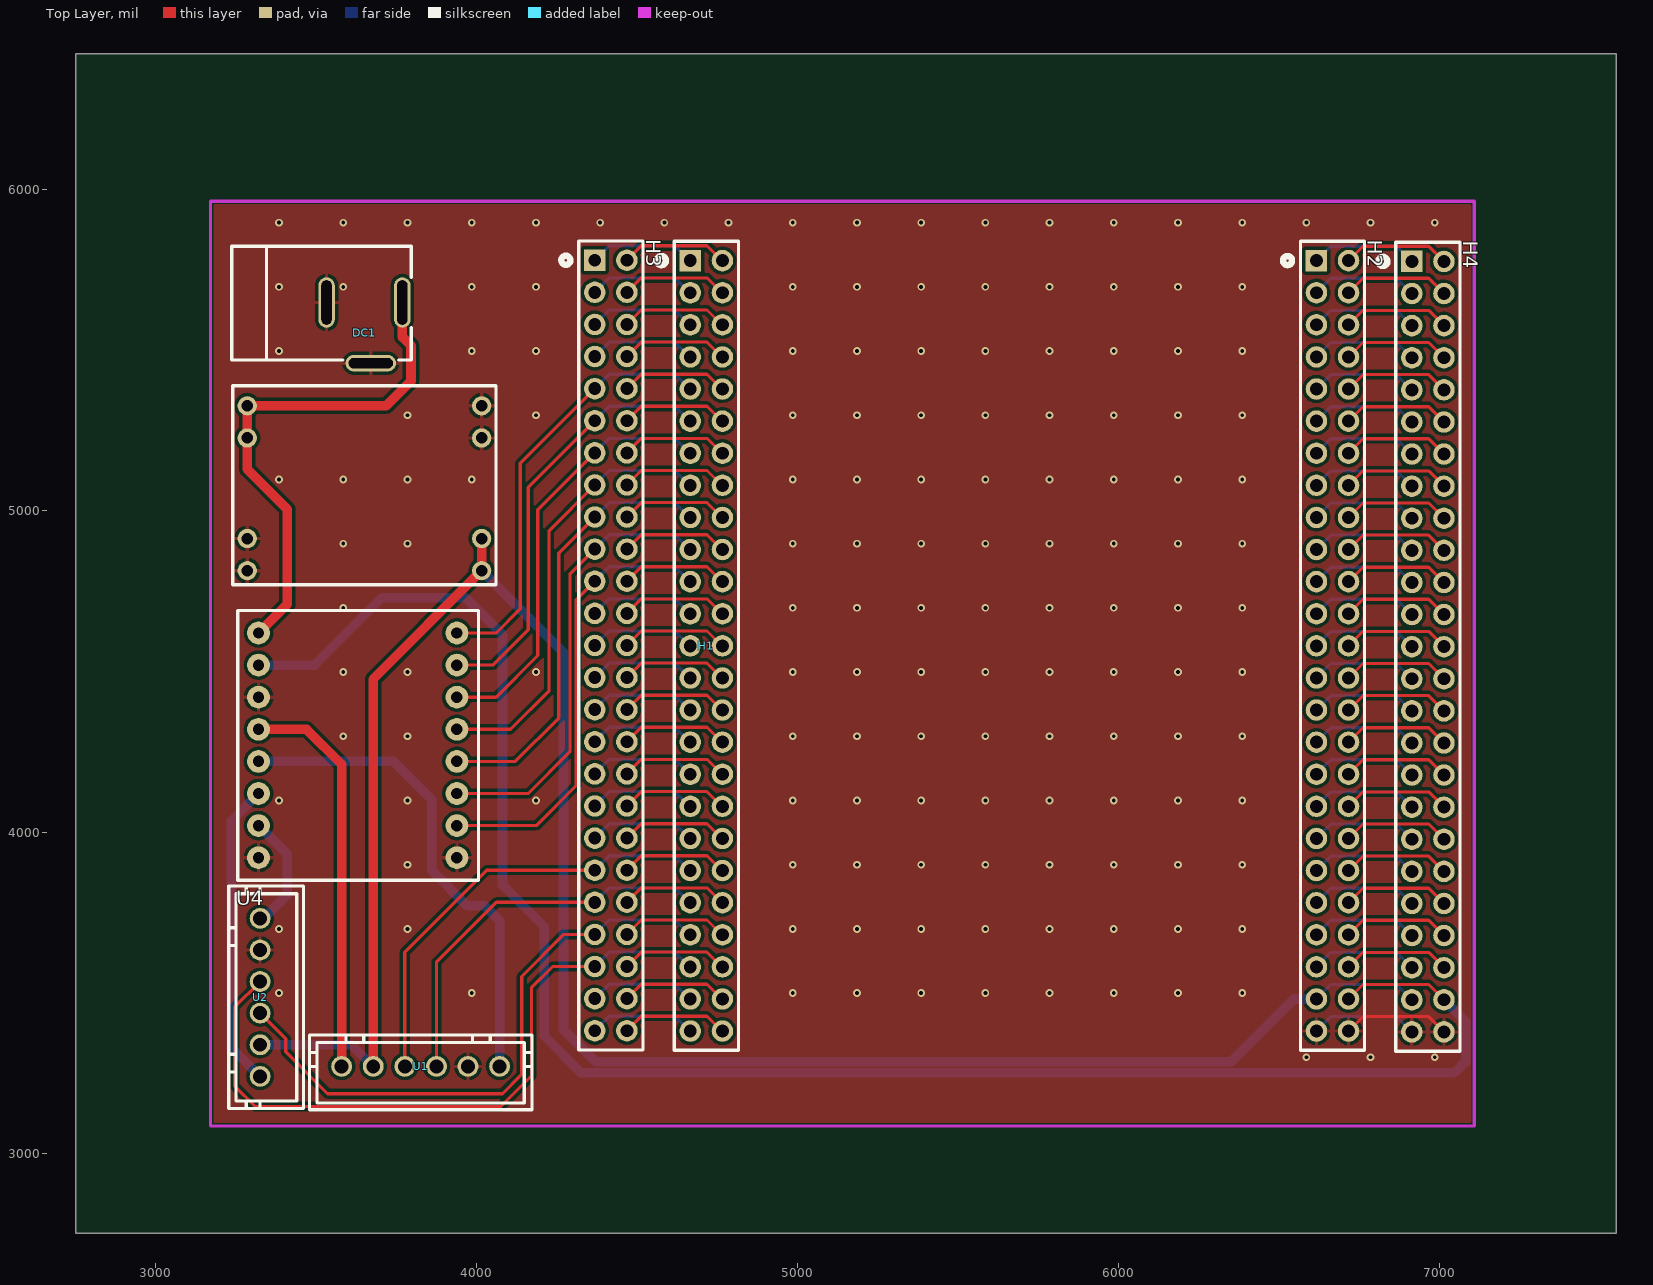
[diagram p0: Top Layer view]
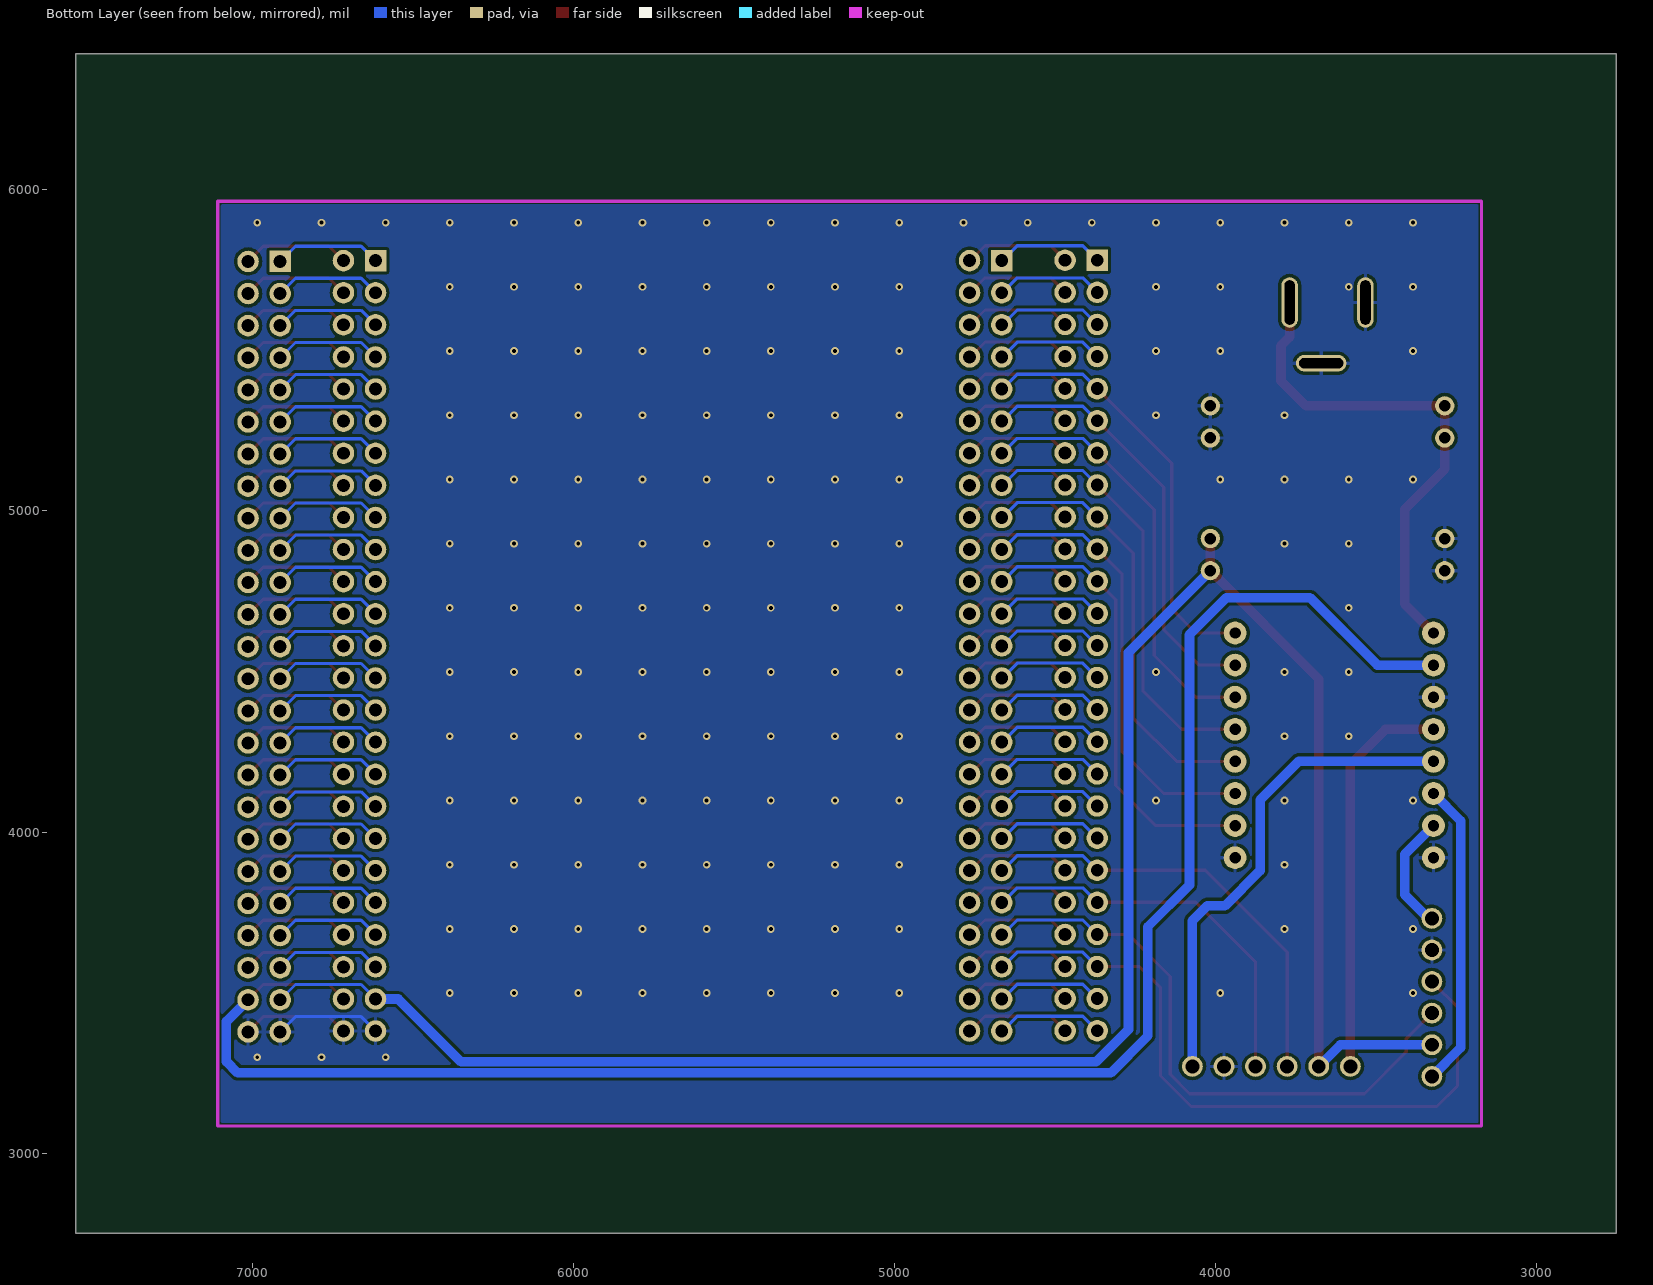
[diagram p1: Bottom Layer view, seen from below]
# Altium PCB MISC89017.pcbdoc
Units mil, origin at the board's own origin, x right, y up, seen from the top; angles counter-clockwise.
Board outline 4800 x 3675 mil, 2 copper layers (Top Layer, Bottom Layer), stack 62.206 mil thick; 8 components, 104 nets, 239 pads, 147 vias.

## Layer stack, top to bottom
Top Solder Mask Layer: solder mask 0.394, Dk 3.3
Top Layer: signal copper 1.379
Dielectric1: surface 59.449, FR4, Dk 4.5
Bottom Layer: signal copper 1.378
Bottom Solder Mask Layer: solder mask 0.394, Dk 3.3

## Board outline
7550,2750 2750,2750 2750,6425 7550,6425

## Design rules (kind name [scope] priority, off if disabled: settings)
BoardOutlineClearance copperThickness2oz_1 [All] p2 off: genericclearance=7.99 ignorepadtopadclearanceinfootprint=FALSE except(0: Arc-SplitContinuation Track-SplitContinuation SMDPad-SplitContinuation THPad-SplitContinuation Via-SplitContinuation Fill-SplitContinuation Region-SplitContinuation Poly-SplitContinuation Text-SplitContinuation Hole-SplitContinuation; 5.98: Arc-CutoutEdge SMDPad-CutoutEdge THPad-CutoutEdge Via-CutoutEdge Fill-CutoutEdge Region-CutoutEdge Text-CutoutEdge; 6.93: Hole-OutlineEdge Hole-CutoutEdge; 10: Poly-OutlineEdge Poly-CutoutEdge; 11.81: Arc-OutlineEdge Track-OutlineEdge SMDPad-OutlineEdge THPad-OutlineEdge Via-OutlineEdge Fill-OutlineEdge Region-OutlineEdge Text-OutlineEdge Track-CutoutEdge)
BoardOutlineClearance copperThickness1oz_1 [All] p4: genericclearance=4.02 ignorepadtopadclearanceinfootprint=FALSE except(0: Arc-SplitContinuation Track-SplitContinuation SMDPad-SplitContinuation THPad-SplitContinuation Via-SplitContinuation Fill-SplitContinuation Region-SplitContinuation Poly-SplitContinuation Text-SplitContinuation Hole-SplitContinuation; 6: SMDPad-CutoutEdge THPad-CutoutEdge Via-CutoutEdge Fill-CutoutEdge Region-CutoutEdge Text-CutoutEdge; 6.93: Hole-OutlineEdge Hole-CutoutEdge; 10: Poly-OutlineEdge Poly-CutoutEdge; 11.8: Arc-OutlineEdge Track-OutlineEdge SMDPad-OutlineEdge THPad-OutlineEdge Via-OutlineEdge Fill-OutlineEdge Region-OutlineEdge Text-OutlineEdge; 11.81: Arc-CutoutEdge Track-CutoutEdge)
Clearance copperThickness2oz [All] p1 off: gap=7.99 ignorepadtopadclearanceinfootprint=FALSE except(5.98: SMDPad-Track SMDPad-SMDPad THPad-Track SMDPad-THPad THPad-THPad Track-Via SMDPad-Via THPad-Via Via-Via Fill-Track Region-Track Fill-SMDPad Region-SMDPad Fill-THPad Region-THPad Fill-Via Region-Via Fill-Fill Fill-Region Region-Region Arc-Track Arc-SMDPad Arc-THPad Arc-Via Fill-Arc Region-Arc Arc-Arc Text-Track SMDPad-Text Text-THPad Text-Via Fill-Text Region-Text Arc-Text Text-Text; 6.93: Hole-Track Hole-SMDPad Hole-THPad Hole-Via Fill-Hole Region-Hole Hole-Arc Hole-Text; 10: Poly-Track Poly-SMDPad Poly-THPad Poly-Via Poly-Fill Poly-Region Poly-Poly Poly-Arc Poly-Text Poly-Hole)
Clearance copperThickness1oz [All] p3: gap=4.02 ignorepadtopadclearanceinfootprint=FALSE except(5.98: SMDPad-Track SMDPad-SMDPad THPad-Track SMDPad-THPad THPad-THPad Track-Via SMDPad-Via THPad-Via Via-Via Fill-Track Region-Track Fill-SMDPad Region-SMDPad Fill-THPad Region-THPad Fill-Via Region-Via Fill-Fill Fill-Region Region-Region; 6: Arc-Track Arc-SMDPad Arc-THPad Arc-Via Fill-Arc Region-Arc Arc-Arc Text-Track SMDPad-Text Text-THPad Text-Via Fill-Text Region-Text Arc-Text Text-Text; 6.93: Hole-Track Hole-SMDPad Hole-THPad Hole-Via Fill-Hole Region-Hole Hole-Arc Hole-Text; 10: Poly-Track Poly-SMDPad Poly-THPad Poly-Via Poly-Fill Poly-Region Poly-Poly Poly-Arc Poly-Text Poly-Hole)
DiffPairsRouting differentialPair [All] p1: maxlimit=6 minlimit=6 mostfreqgap=6 toplayer_minwidth=5 toplayer_prefwidth=10 toplayer_maxwidth=100 toplayer_mingap=6 toplayer_prefgap=6 toplayer_maxgap=6 bottomlayer_minwidth=5 bottomlayer_prefwidth=10 bottomlayer_maxwidth=100 bottomlayer_mingap=6 bottomlayer_prefgap=6 bottomlayer_maxgap=6 maxuncoupledlength=10
HoleToHoleClearance otherClearance [All] p1: gap=11.81 allowstackedmicrovias=TRUE
Length netLength [All] p1: minlimit=0 maxlimit=0
MatchedLengths netLengthTolerance [All] p1: tolerance=1000
PasteMaskExpansion pasteMaskExpansion [All] p1: expansion=0
PlaneConnect innerPlane [All] p1: planeconnectstyle=Relief reliefexpansion=20 reliefentries=4 reliefconductorwidth=10 reliefairgap=10
PolygonConnect copperRegion [(InNet('GND'))] p1: connectstyle=Relief reliefconductorwidth=10 reliefentries=4 polygonreliefangle="90 Angle" airgapwidth=10 via.connectstyle=Relief via.reliefconductorwidth=10 via.reliefentries=4 via.polygonreliefangle="90 Angle" via.airgapwidth=10
RoutingVias viaSize [All] p1: holewidth=12.01 width=24.02 viastyle="Through Hole" minholewidth=11.81 minwidth=19.68 maxholewidth=248.03 maxwidth=393.7
SolderMaskExpansion solderMaskExpansion [IsVia] p1: expansion=-1000 istentingtop=TRUE
SolderMaskExpansion solderMaskExpansion [All] p2: expansion=2 istentingtop=FALSE
Width copperThickness2oz_2 [All] p1 off: maxlimit=100 minlimit=8 preferedwidth=10
Width copperThickness1oz_2 [All] p2: maxlimit=100 minlimit=5 preferedwidth=10

## Components (designator, comment, footprint, x,y, rotation, side; value= is the part's Value field where it differs from the comment)
DC1 "" DC-2.0 3645,5660 r180 top
H1 "2.54-2*25" HDR-TH_50P-P2.54-V-F-R2-C25-S2.54-1 4715,4580 r270 top
H2 "2.54-2*25" HDR-TH_50P-P2.54-V-F-R2-C25-S2.54-1 6665.41,4580 r270 top
H3 "2.54-2*25" HDR-TH_50P-P2.54-V-F-R2-C25-S2.54-1 4417.5,4581.08 r270 top
H4 "2.54-2*25" HDR-TH_50P-P2.54-V-F-R2-C25-S2.54-1 6962.5,4577.41 r270 top
U1 "XH2.54-6P through-hole" CONN-TH_XH2.54-6P 3825,3270 r0 top
U2 "XH2.54-6P through-hole" CONN-TH_XH2.54-6P 3325,3485 r90 top
U4 "" tb6612 3320,4620 r0 top

## Footprints (in the part's own frame and the unit in brackets; to place one, negate y for a bottom-side part, rotate by r counter-clockwise, add the part's x,y. Pads: shape width x height; smd on the part's side, far side on the other; paste and mask are expansions set on the pad)
CONN-TH_XH2.54-6P [mm]
  round 1.65 hole 1.1 paste+0 mask+0.05: 1(-6.25,0) 2(-3.75,0) 3(-1.25,0) 4(1.25,0) 5(3.75,0) 6(6.25,0)
  silkscreen extent -8.8,-3.43 8.8,2.47
DC-2.0 [mil]
  oval 157.5x51.2 hole 31.5 slot 137.8 at 0 deg paste+0 mask+2: 2(-24.7,199.5)
  oval 51.2x157.5 hole 31.5 slot 137.8 at 90 deg paste+0 mask+2: 3(113.1,10.5) 4(-123.1,10.5)
  silkscreen extent -151,-165 408,190
HDR-TH_50P-P2.54-V-F-R2-C25-S2.54-1 [mm]
  rect 1.7x1.7 hole 1.02: 1(-30.48,-1.27)
  round 1.7 hole 1.02: 2(-30.48,1.27) 3(-27.94,-1.27) 4(-27.94,1.27) 5(-25.4,-1.27) 6(-25.4,1.27) 7(-22.86,-1.27) 8(-22.86,1.27) 9(-20.32,-1.27) 10(-20.32,1.27) 11(-17.78,-1.27) 12(-17.78,1.27) 13(-15.24,-1.27) 14(-15.24,1.27) 15(-12.7,-1.27) 16(-12.7,1.27) 17(-10.16,-1.27) 18(-10.16,1.27) 19(-7.62,-1.27) 20(-7.62,1.27) 21(-5.08,-1.27) 22(-5.08,1.27) 23(-2.54,-1.27) 24(-2.54,1.27) 25(0,-1.27) 26(0,1.27) 27(2.54,-1.27) 28(2.54,1.27) 29(5.08,-1.27) 30(5.08,1.27) 31(7.62,-1.27) 32(7.62,1.27) 33(10.16,-1.27) 34(10.16,1.27) 35(12.7,-1.27) 36(12.7,1.27) 37(15.24,-1.27) 38(15.24,1.27) 39(17.78,-1.27) 40(17.78,1.27) 41(20.32,-1.27) 42(20.32,1.27) 43(22.86,-1.27) 44(22.86,1.27) 45(25.4,-1.27) 46(25.4,1.27) 47(27.94,-1.27) 48(27.94,1.27) 49(30.48,-1.27) 50(30.48,1.27)
  silkscreen extent -32,-3.91 32,2.54
tb6612 [mm]
  round 1.8 hole 0.9: 1(0,0) 2(0,-2.54) 3(0,-5.08) 4(0,-7.62) 5(0,-10.16) 6(0,-12.7) 7(0,-15.24) 8(0,-17.78) 9(15.697,-17.78) 10(15.697,-15.24) 11(15.697,-12.7) 12(15.697,-10.16) 13(15.697,-7.62) 14(15.697,-5.08) 15(15.697,-2.54) 16(15.697,0)
  silkscreen extent -1.65,-19.56 17.4,1.78

## Free pads (board coordinates)
  round 60 hole 36: 1(3285.04,5327.53) 1(4015.04,5227.53) 2(3285.04,5227.53) 3(3285.04,4914.14) 4(3285.04,4814.13) 5(4015.04,4914.14) 6(4015.04,4814.13) 7(4015.04,5327.53)

## Via types
v1: diameter 24.02, hole 12, Top Layer to Bottom Layer, 147 vias

## Nets (pads, with @x,y where several pads share a name; then routed paths per layer and width w, separated by ;. In a path a pad name is that pad's centre, name@x,y a point inside that pad or via, vN(x,y) a via of type N, cw(c..) or ccw(c..) an arc to the next point about the centre after c; other vN are vias at no path point)
12V: DC1.4 pad.1@3285.04,5327.53 pad.2 U4.1 | length 1594.3
  Top Layer w30: U4.1 3410,4710 3410,5005 3285.04,5129.96 pad.2 3285.04,5327.53 3717.53,5327.53 3795,5405 3795,5515 3768.1,5541.9 DC1.4
$1N50: H1.21 H3.21 U4.10 | length 1419.1
  Top Layer w10: U4.10 4185,4020 4310,4145 4310,4723.58 H3.21
  Bottom Layer w10: H3.21 4412.5,4826.08 4617.01,4826.08 H1.21@4664.59,4778.49
$1N51: H1.19 H3.19 U4.11 | length 1404.5
  Top Layer w10: U4.11 4160,4120 4290,4250 4290,4803.58 H3.19
  Bottom Layer w10: H3.19 4412.5,4926.08 4617.01,4926.08 H1.19@4664.59,4878.49
$1N52: H1.17 H3.17 U4.12 | length 1381
  Top Layer w10: U4.12 4120,4220 4255,4355 4255,4868.58 H3.17
  Bottom Layer w10: H3.17 4412.5,5026.08 4617.01,5026.08 H1.17@4664.59,4978.49
$1N53: H1.15 H3.15 U4.13 | length 1372.3
  Top Layer w10: U4.13 4105,4320 4225,4440 4225,4938.58 H3.15
  Bottom Layer w10: H3.15 4412.5,5126.08 4617.01,5126.08 H1.15@4664.59,5078.49
$1N54: H1.13 H3.13 U4.14 | length 1345.9
  Top Layer w10: U4.14 4060,4420 4190,4550 4190,5003.58 H3.13
  Bottom Layer w10: H3.13 4412.5,5226.08 4617.01,5226.08 H1.13@4664.59,5178.49
$1N55: H1.11 H3.11 U4.15 | length 1340
  Top Layer w10: U4.15 4050,4520 4160,4630 4160,5073.58 H3.11
  Bottom Layer w10: H3.11 4412.5,5326.08 4617.01,5326.08 H1.11@4664.59,5278.49
$1N56: H1.9 H3.9 U4.16 | length 1345.9
  Top Layer w10: U4.16 4060,4620 4135,4695 4135,5148.58 H3.9
  Bottom Layer w10: H3.9 4412.5,5426.08 4617.01,5426.08 H1.9@4664.59,5378.49
$1N61: U1.1 U4.4 | length 1245.1
  Top Layer w30: U4.4 3470,4320 3578.94,4211.06 U1.1
$1N64: U2.6 U4.7 | length 367.9
  Bottom Layer w30: U4.7 3410,3930 3410,3805 3336.06,3731.06 U2.6
$1N66: H1.1 H3.1 | length 335.4
  Bottom Layer w10: H3.1 4412.5,5826.08 4617.01,5826.08 H1.1@4664.59,5778.49
$1N67: H1.50 H3.50 | length 335.4
  Top Layer w10: H3.50 4512.5,3426.08 4717.01,3426.08 H1.50@4764.59,3378.49
$1N68: H1.3 H3.3 | length 335.4
  Bottom Layer w10: H3.3 4412.5,5726.08 4617.01,5726.08 H1.3@4664.59,5678.49
$1N69: H1.48 H3.48 | length 335.4
  Top Layer w10: H3.48 4512.5,3526.08 4717.01,3526.08 H1.48@4764.59,3478.49
$1N70: H1.5 H3.5 | length 335.4
  Bottom Layer w10: H3.5 4412.5,5626.08 4617.01,5626.08 H1.5@4664.59,5578.49
$1N71: H1.46 H3.46 | length 335.4
  Top Layer w10: H3.46 4512.5,3626.08 4717.01,3626.08 H1.46@4764.59,3578.49
$1N72: H1.7 H3.7 | length 335.4
  Bottom Layer w10: H3.7 4412.5,5526.08 4617.01,5526.08 H1.7@4664.59,5478.49
$1N73: H1.44 H3.44 | length 335.4
  Top Layer w10: H3.44 4512.5,3726.08 4717.01,3726.08 H1.44@4764.59,3678.49
$1N74: H1.42 H3.42 | length 335.4
  Top Layer w10: H3.42 4512.5,3826.08 4717.01,3826.08 H1.42@4764.59,3778.49
$1N75: H1.40 H3.40 | length 335.4
  Top Layer w10: H3.40 4512.5,3926.08 4717.01,3926.08 H1.40@4764.59,3878.49
$1N76: H1.38 H3.38 | length 335.4
  Top Layer w10: H3.38 4512.5,4026.08 4717.01,4026.08 H1.38@4764.59,3978.49
$1N77: H1.36 H3.36 | length 335.4
  Top Layer w10: H3.36 4512.5,4126.08 4717.01,4126.08 H1.36@4764.59,4078.49
$1N78: H1.34 H3.34 | length 335.4
  Top Layer w10: H3.34 4512.5,4226.08 4717.01,4226.08 H1.34@4764.59,4178.49
$1N79: H1.32 H3.32 | length 335.4
  Top Layer w10: H3.32 4512.5,4326.08 4717.01,4326.08 H1.32@4764.59,4278.49
$1N80: H1.30 H3.30 | length 335.4
  Top Layer w10: H3.30 4512.5,4426.08 4717.01,4426.08 H1.30@4764.59,4378.49
$1N81: H1.23 H3.23 | length 335.4
  Bottom Layer w10: H3.23 4412.5,4726.08 4617.01,4726.08 H1.23@4664.59,4678.49
$1N82: H1.28 H3.28 | length 335.4
  Top Layer w10: H3.28 4512.5,4526.08 4717.01,4526.08 H1.28@4764.59,4478.49
$1N83: H1.25 H3.25 | length 335.4
  Bottom Layer w10: H3.25 4412.5,4626.08 4617.01,4626.08 H1.25@4664.59,4578.49
$1N84: H1.26 H3.26 | length 335.4
  Top Layer w10: H3.26 4512.5,4626.08 4717.01,4626.08 H1.26@4764.59,4578.49
$1N85: H1.27 H3.27 | length 335.4
  Bottom Layer w10: H3.27 4412.5,4526.08 4617.01,4526.08 H1.27@4664.59,4478.49
$1N86: H1.24 H3.24 | length 335.4
  Top Layer w10: H3.24 4512.5,4726.08 4717.01,4726.08 H1.24@4764.59,4678.49
$1N87: H1.29 H3.29 | length 335.4
  Bottom Layer w10: H3.29 4412.5,4426.08 4617.01,4426.08 H1.29@4664.59,4378.49
$1N88: H1.22 H3.22 | length 335.4
  Top Layer w10: H3.22 4512.5,4826.08 4717.01,4826.08 H1.22@4764.59,4778.49
$1N89: H1.31 H3.31 | length 335.4
  Bottom Layer w10: H3.31 4412.5,4326.08 4617.01,4326.08 H1.31@4664.59,4278.49
$1N90: H1.20 H3.20 | length 335.4
  Top Layer w10: H3.20 4512.5,4926.08 4717.01,4926.08 H1.20@4764.59,4878.49
$1N91: H1.33 H3.33 | length 335.4
  Bottom Layer w10: H3.33 4412.5,4226.08 4617.01,4226.08 H1.33@4664.59,4178.49
$1N92: H1.18 H3.18 | length 335.4
  Top Layer w10: H3.18 4512.5,5026.08 4717.01,5026.08 H1.18@4764.59,4978.49
$1N93: H1.35 H3.35 | length 335.4
  Bottom Layer w10: H3.35 4412.5,4126.08 4617.01,4126.08 H1.35@4664.59,4078.49
$1N94: H1.16 H3.16 | length 335.4
  Top Layer w10: H3.16 4512.5,5126.08 4717.01,5126.08 H1.16@4764.59,5078.49
$1N95: H1.37 H3.37 | length 335.4
  Bottom Layer w10: H3.37 4412.5,4026.08 4617.01,4026.08 H1.37@4664.59,3978.49
$1N96: H1.14 H3.14 | length 335.4
  Top Layer w10: H3.14 4512.5,5226.08 4717.01,5226.08 H1.14@4764.59,5178.49
$1N97: H1.39 H3.39 U1.3 | length 1388.7
  Top Layer w10: U1.3 3775.79,3625.79 4031.08,3881.08 H3.39
  Bottom Layer w10: H3.39 4412.5,3926.08 4617.01,3926.08 H1.39@4664.59,3878.49
$1N98: H1.12 H3.12 | length 335.4
  Top Layer w10: H3.12 4512.5,5326.08 4717.01,5326.08 H1.12@4764.59,5278.49
$1N99: H1.41 H3.41 U1.4 | length 1230.3
  Top Layer w10: U1.4 3874.21,3594.21 4061.08,3781.08 H3.41
  Bottom Layer w10: H3.41 4412.5,3826.08 4617.01,3826.08 H1.41@4664.59,3778.49
$1N100: H1.10 H3.10 | length 335.4
  Top Layer w10: H3.10 4512.5,5426.08 4717.01,5426.08 H1.10@4764.59,5378.49
$1N101: H1.43 H3.43 U2.3 | length 1889.9
  Top Layer w10: U2.3 3405,3355.79 3405,3315 3535,3185 4080,3185 4140,3245 4140,3550 4271.08,3681.08 H3.43
  Bottom Layer w10: H3.43 4412.5,3726.08 4617.01,3726.08 H1.43@4664.59,3678.49
$1N102: H1.8 H3.8 | length 335.4
  Top Layer w10: H3.8 4512.5,5526.08 4717.01,5526.08 H1.8@4764.59,5478.49
$1N103: H1.45 H3.45 U2.4 | length 2183.9
  Top Layer w10: U2.4 3245,3454.21 3245,3210 3310,3145 4075,3145 4170,3240 4170,3515 4236.08,3581.08 H3.45
  Bottom Layer w10: H3.45 4412.5,3626.08 4617.01,3626.08 H1.45@4664.59,3578.49
$1N104: H1.6 H3.6 | length 335.4
  Top Layer w10: H3.6 4512.5,5626.08 4717.01,5626.08 H1.6@4764.59,5578.49
$1N105: H1.47 H3.47 | length 335.4
  Bottom Layer w10: H3.47 4412.5,3526.08 4617.01,3526.08 H1.47@4664.59,3478.49
$1N106: H1.4 H3.4 | length 335.4
  Top Layer w10: H3.4 4512.5,5726.08 4717.01,5726.08 H1.4@4764.59,5678.49
$1N107: H1.49 H3.49 | length 335.4
  Bottom Layer w10: H3.49 4412.5,3426.08 4617.01,3426.08 H1.49@4664.59,3378.49
$1N108: H1.2 H3.2 | length 335.4
  Top Layer w10: H3.2 4512.5,5826.08 4717.01,5826.08 H1.2@4764.59,5778.49
$1N109: H2.1 H4.1 | length 335.4
  Bottom Layer w10: H2.1 6660.41,5825 6864.91,5825 H4.1
$1N110: H2.3 H4.3 | length 335.4
  Bottom Layer w10: H2.3 6660.41,5725 6864.91,5725 H4.3
$1N111: H2.5 H4.5 | length 335.4
  Bottom Layer w10: H2.5 6660.41,5625 6864.91,5625 H4.5
$1N112: H2.46 H4.46 | length 335.4
  Top Layer w10: H2.46 6760.41,3625 6964.91,3625 H4.46
$1N113: H2.7 H4.7 | length 335.4
  Bottom Layer w10: H2.7 6660.41,5525 6864.91,5525 H4.7
$1N114: H2.44 H4.44 | length 335.4
  Top Layer w10: H2.44 6760.41,3725 6964.91,3725 H4.44
$1N115: H2.9 H4.9 | length 335.4
  Bottom Layer w10: H2.9 6660.41,5425 6864.91,5425 H4.9
$1N116: H2.42 H4.42 | length 335.4
  Top Layer w10: H2.42 6760.41,3825 6964.91,3825 H4.42
$1N117: H2.11 H4.11 | length 335.4
  Bottom Layer w10: H2.11 6660.41,5325 6864.91,5325 H4.11
$1N118: H2.40 H4.40 | length 335.4
  Top Layer w10: H2.40 6760.41,3925 6964.91,3925 H4.40
$1N119: H2.13 H4.13 | length 335.4
  Bottom Layer w10: H2.13 6660.41,5225 6864.91,5225 H4.13
$1N120: H2.38 H4.38 | length 335.4
  Top Layer w10: H2.38 6760.41,4025 6964.91,4025 H4.38
$1N121: H2.15 H4.15 | length 335.4
  Bottom Layer w10: H2.15 6660.41,5125 6864.91,5125 H4.15
$1N122: H2.36 H4.36 | length 335.4
  Top Layer w10: H2.36 6760.41,4125 6964.91,4125 H4.36
$1N123: H2.17 H4.17 | length 335.4
  Bottom Layer w10: H2.17 6660.41,5025 6864.91,5025 H4.17
$1N124: H2.34 H4.34 | length 335.4
  Top Layer w10: H2.34 6760.41,4225 6964.91,4225 H4.34
$1N125: H2.19 H4.19 | length 335.4
  Bottom Layer w10: H2.19 6660.41,4925 6864.91,4925 H4.19
$1N126: H2.32 H4.32 | length 335.4
  Top Layer w10: H2.32 6760.41,4325 6964.91,4325 H4.32
$1N127: H2.21 H4.21 | length 335.4
  Bottom Layer w10: H2.21 6660.41,4825 6864.91,4825 H4.21
$1N128: H2.30 H4.30 | length 335.4
  Top Layer w10: H2.30 6760.41,4425 6964.91,4425 H4.30
$1N129: H2.23 H4.23 | length 335.4
  Bottom Layer w10: H2.23 6660.41,4725 6864.91,4725 H4.23
$1N130: H2.28 H4.28 | length 335.4
  Top Layer w10: H2.28 6760.41,4525 6964.91,4525 H4.28
$1N131: H2.25 H4.25 | length 335.4
  Bottom Layer w10: H2.25 6660.41,4625 6864.91,4625 H4.25
$1N132: H2.26 H4.26 | length 335.4
  Top Layer w10: H2.26 6760.41,4625 6964.91,4625 H4.26
$1N133: H2.27 H4.27 | length 335.4
  Bottom Layer w10: H2.27 6660.41,4525 6864.91,4525 H4.27
$1N134: H2.24 H4.24 | length 335.4
  Top Layer w10: H2.24 6760.41,4725 6964.91,4725 H4.24
$1N135: H2.29 H4.29 | length 335.4
  Bottom Layer w10: H2.29 6660.41,4425 6864.91,4425 H4.29
$1N136: H2.22 H4.22 | length 335.4
  Top Layer w10: H2.22 6760.41,4825 6964.91,4825 H4.22
$1N137: H2.31 H4.31 | length 335.4
  Bottom Layer w10: H2.31 6660.41,4325 6864.91,4325 H4.31
$1N138: H2.20 H4.20 | length 335.4
  Top Layer w10: H2.20 6760.41,4925 6964.91,4925 H4.20
$1N139: H2.33 H4.33 | length 335.4
  Bottom Layer w10: H2.33 6660.41,4225 6864.91,4225 H4.33
$1N140: H2.18 H4.18 | length 335.4
  Top Layer w10: H2.18 6760.41,5025 6964.91,5025 H4.18
$1N141: H2.35 H4.35 | length 335.4
  Bottom Layer w10: H2.35 6660.41,4125 6864.91,4125 H4.35
$1N142: H2.16 H4.16 | length 335.4
  Top Layer w10: H2.16 6760.41,5125 6964.91,5125 H4.16
$1N143: H2.37 H4.37 | length 335.4
  Bottom Layer w10: H2.37 6660.41,4025 6864.91,4025 H4.37
$1N144: H2.14 H4.14 | length 335.4
  Top Layer w10: H2.14 6760.41,5225 6964.91,5225 H4.14
$1N145: H2.39 H4.39 | length 335.4
  Bottom Layer w10: H2.39 6660.41,3925 6864.91,3925 H4.39
$1N146: H2.12 H4.12 | length 335.4
  Top Layer w10: H2.12 6760.41,5325 6964.91,5325 H4.12
$1N147: H2.41 H4.41 | length 335.4
  Bottom Layer w10: H2.41 6660.41,3825 6864.91,3825 H4.41
$1N148: H2.10 H4.10 | length 335.4
  Top Layer w10: H2.10 6760.41,5425 6964.91,5425 H4.10
$1N149: H2.43 H4.43 | length 335.4
  Bottom Layer w10: H2.43 6660.41,3725 6864.91,3725 H4.43
$1N150: H2.8 H4.8 | length 335.4
  Top Layer w10: H2.8 6760.41,5525 6964.91,5525 H4.8
$1N151: H2.45 H4.45 | length 335.4
  Bottom Layer w10: H2.45 6660.41,3625 6864.91,3625 H4.45
$1N152: H2.6 H4.6 | length 335.4
  Top Layer w10: H2.6 6760.41,5625 6964.91,5625 H4.6
$1N153: H2.4 H4.4 | length 335.4
  Top Layer w10: H2.4 6760.41,5725 6964.91,5725 H4.4
$1N154: H2.2 H4.2 | length 335.4
  Top Layer w10: H2.2 6760.41,5825 6964.91,5825 H4.2
$1N155: U1.6 U4.5 | length 1539.3
  Bottom Layer w30: U4.5 3740,4220 3860,4100 3860,3880 3970,3770 4025,3770 4071.06,3723.94 U1.6
$1N156: U2.1 U4.6 | length 953.5
  Bottom Layer w30: U4.6 3235,4035 3235,3328.94 U2.1
+5V: H2.47 H4.47 pad.5 pad.6 U1.2 U2.2 | length 6502.9
  Top Layer w30: U1.2 3677.36,4476.45 pad.6 pad.5
  Bottom Layer w10: H2.47 6660.41,3525 6864.91,3525 H4.47
  Bottom Layer w30: U2.2 3610,3337.36 U1.2 ; pad.6 4270,4559.17 4270,3385 4370.98,3284.02 6349.02,3284.02 6545,3480 H2.47
GND: DC1.2 DC1.3 H2.49 H2.50 H4.49 H4.50 pad.1@4015.04,5227.53 pad.3 pad.4 pad.7 U1.5 U2.5 U4.3 U4.8 U4.9 | length 670.9
  Top Layer w10: H2.50 6760.41,3425 6964.91,3425 H4.50
  Bottom Layer w10: H2.49 6660.41,3425 6864.91,3425 H4.49
  other v1: 6584.1,3298.25 6784.1,3298.25 6984.1,3298.25 3384.1,3498.25 3984.1,3498.25 4984.1,3498.25 5184.1,3498.25 5384.1,3498.25 5584.1,3498.25 5784.1,3498.25 5984.1,3498.25 6184.1,3498.25 6384.1,3498.25 3384.1,3698.25 3784.1,3698.25 4984.1,3698.25 5184.1,3698.25 5384.1,3698.25 5584.1,3698.25 5784.1,3698.25 5984.1,3698.25 6184.1,3698.25 6384.1,3698.25 3784.1,3898.25 4984.1,3898.25 5184.1,3898.25 5384.1,3898.25 5584.1,3898.25 5784.1,3898.25 5984.1,3898.25 6184.1,3898.25 6384.1,3898.25 3384.1,4098.25 3784.1,4098.25 4184.1,4098.25 4984.1,4098.25 5184.1,4098.25 5384.1,4098.25 5584.1,4098.25 5784.1,4098.25 5984.1,4098.25 6184.1,4098.25 6384.1,4098.25 3584.1,4298.25 3784.1,4298.25 4984.1,4298.25 5184.1,4298.25 5384.1,4298.25 5584.1,4298.25 5784.1,4298.25 5984.1,4298.25 6184.1,4298.25 6384.1,4298.25 3584.1,4498.25 3784.1,4498.25 4184.1,4498.25 4984.1,4498.25 5184.1,4498.25 5384.1,4498.25 5584.1,4498.25 5784.1,4498.25 5984.1,4498.25 6184.1,4498.25 6384.1,4498.25 3584.1,4698.25 4984.1,4698.25 5184.1,4698.25 5384.1,4698.25 5584.1,4698.25 5784.1,4698.25 5984.1,4698.25 6184.1,4698.25 6384.1,4698.25 3584.1,4898.25 3784.1,4898.25 4984.1,4898.25 5184.1,4898.25 5384.1,4898.25 5584.1,4898.25 5784.1,4898.25 5984.1,4898.25 6184.1,4898.25 6384.1,4898.25 3384.1,5098.25 3584.1,5098.25 3784.1,5098.25 3984.1,5098.25 4984.1,5098.25 5184.1,5098.25 5384.1,5098.25 5584.1,5098.25 5784.1,5098.25 5984.1,5098.25 6184.1,5098.25 6384.1,5098.25 3784.1,5298.25 4184.1,5298.25 4984.1,5298.25 5184.1,5298.25 5384.1,5298.25 5584.1,5298.25 5784.1,5298.25 5984.1,5298.25 6184.1,5298.25 6384.1,5298.25 3384.1,5498.25 3984.1,5498.25 4184.1,5498.25 4984.1,5498.25 5184.1,5498.25 5384.1,5498.25 5584.1,5498.25 5784.1,5498.25 5984.1,5498.25 6184.1,5498.25 6384.1,5498.25 3384.1,5698.25 3584.1,5698.25 3984.1,5698.25 4184.1,5698.25 4984.1,5698.25 5184.1,5698.25 5384.1,5698.25 5584.1,5698.25 5784.1,5698.25 5984.1,5698.25 6184.1,5698.25 6384.1,5698.25 3384.1,5898.25 3584.1,5898.25 3784.1,5898.25 3984.1,5898.25 4184.1,5898.25 4384.1,5898.25 4584.1,5898.25 4784.1,5898.25 4984.1,5898.25 5184.1,5898.25 5384.1,5898.25 5584.1,5898.25 5784.1,5898.25 5984.1,5898.25 6184.1,5898.25 6384.1,5898.25 6584.1,5898.25 6784.1,5898.25 6984.1,5898.25
VCC: H2.48 H4.48 U4.2 | length 5686.6
  Top Layer w10: H2.48 6760.41,3525 6964.91,3525 H4.48
  Bottom Layer w30: U4.2 3495,4520 3705,4730 3965,4730 4080,4615 4080,3835 4210,3705 4210,3365 4325,3250 7045,3250 7080.21,3285.21 7080.21,3409.71 H4.48

## Polygon pours and split planes (outlines as drawn)
GND on Top Layer (solid, remove dead copper, pour order 0): 3020,6175 3020,3050 7300,3050 7300,6175
GND on Bottom Layer (solid, remove dead copper, pour order 2): 3000,6105 3000,3000 7115,3000 7115,6105

## Keep-outs
Board Outline Layer:
  lines w10: 3170,3084.15 3170,5965 7107.01,5965 7107.01,3084.15 3170,3084.15

## Silkscreen, mask and mechanical layers (free items; w line width, h text height)
Top Silkscreen Layer:
  lines w10: 3240,4770 3240,5390 4060,5390 4060,4770 3240,4770